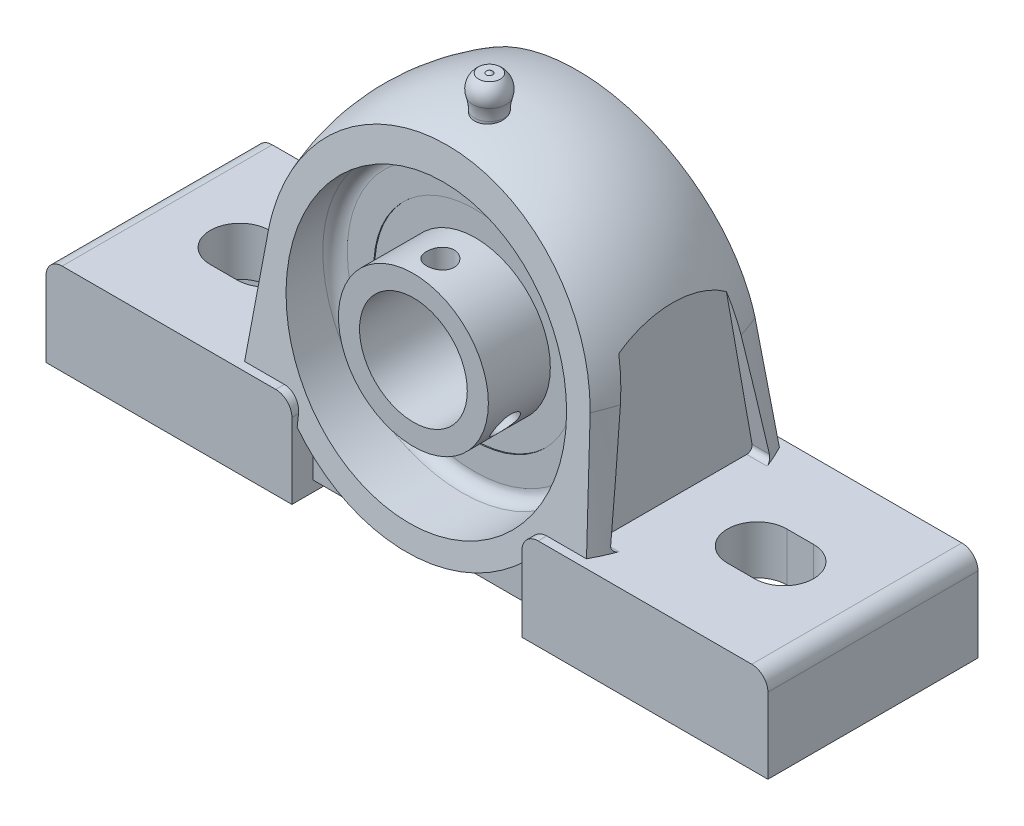
from build123d import *

# Parameters (mm, degrees)
EXTRUDE_984_DEPTH             = 84.85
CUT_EXTRUDE_1_DEPTH           = 55.135249472
CUT_EXTRUDE_1_DEPTH_BACK      = 55.135249472
SKETCH_5_OUTSIDE_W            = 60.452
SKETCH_5_OUTSIDE_H            = 88.062
EXTRUDE_4_REACH               = 60.025
EXTRUDE_4_DIRECTION_2_REACH   = 60.025
EXTRUDE_1_DEPTH               = 19.5
EXTRUDE_1_DEPTH_BACK          = 19.5
CUT_EXTRUDE_3_DEPTH           = 101.761654379
CUT_EXTRUDE_4_DEPTH           = 7.99
CUT_EXTRUDE_4_DRAFT           = -1
CUT_EXTRUDE_4_PROFILE_2_DEPTH = 7.99
CUT_EXTRUDE_4_PROFILE_2_DRAFT = -1
PATTERN_CIRCULAR_1_COUNT      = 12
SKETCH_14_W                   = 31
SKETCH_14_H                   = 3.915
SKETCH_16_W                   = 2.567
SKETCH_16_H                   = 6.115
SKETCH_15_W                   = 0.1
SKETCH_15_H                   = 5.145
PATTERN_CIRCULAR_2_COUNT      = 2
PATTERN_CIRCULAR_2_ANGLE      = 120
CUT_EXTRUDE_START             = 29.81311
CUT_EXTRUDE_5_DEPTH           = 8.58689
CUT_EXTRUDE_START_2           = -38.4
CUT_EXTRUDE_6_DEPTH           = 8.49652


with BuildPart() as part:
    # 草图1 → Extrude 984 (new body)
    with BuildSketch(Plane(origin=(0, -31.3, 0), x_dir=(-1, 0, 0), z_dir=(0, 1, 0))):
        with BuildLine():
            Line((-33.636057661, 18.525), (33.636057661, 18.525))
            ThreePointArc((33.636057661, 18.525), (38.4, 0), (33.636057661, -18.525))
            Line((33.636057661, -18.525), (-33.636057661, -18.525))
            ThreePointArc((-33.636057661, -18.525), (-38.4, 0), (-33.636057661, 18.525))
        make_face()
    extrude(amount=EXTRUDE_984_DEPTH)

    # 切除-扫描1: sweep along a path in 草图3
    with BuildLine(Plane.XY) as sweep_1_path:
        Line((-38.4, -31.3), (-32.994675679, 4.923512654))
        ThreePointArc((-32.994675679, 4.923512654), (0, 33.36), (32.994675679, 4.923512654))
        Line((32.994675679, 4.923512654), (38.4, -31.3))
    # 草图2 → 切除-扫描1 (sweep, cut)
    with BuildSketch(Plane(origin=(0, -31.3, 0), x_dir=(-1, 0, 0), z_dir=(0, 1, 0))):
        with BuildLine():
            Line((-33.636057661, 18.525), (-123.25, 18.525))
            Line((-123.25, 18.525), (-123.25, -18.525))
            Line((-123.25, -18.525), (-33.636057661, -18.525))
            ThreePointArc((-33.636057661, -18.525), (-38.4, 0), (-33.636057661, 18.525))
        make_face()
    sweep(path=sweep_1_path.line, mode=Mode.SUBTRACT)

    # 草图5 outside → 切除-拉伸1 (cut, two sides: drawn at the far end of the back side and taken through both)
    with BuildSketch(Plane(origin=(0, 0, 0), x_dir=(0, 0, -1), z_dir=(1, 0, 0)).offset(-CUT_EXTRUDE_1_DEPTH_BACK)):
        with Locations((0, 1.03)):
            Rectangle(SKETCH_5_OUTSIDE_W, SKETCH_5_OUTSIDE_H)
        Polygon((11.7, 34.36), (18.525, -21.38), (15.6, -21.38), (15.6, -34.3), (-15.6, -34.3), (-15.6, -21.38), (-18.525, -21.38), (-11.7, 34.36), align=None, mode=Mode.SUBTRACT)
    extrude(amount=CUT_EXTRUDE_1_DEPTH + CUT_EXTRUDE_1_DEPTH_BACK, mode=Mode.SUBTRACT)

    # 草图6 → 切除-旋转2 (revolve, cut)
    with BuildSketch(Plane(origin=(0, 0, 0), x_dir=(0, 0, -1), z_dir=(1, 0, 0)), mode=Mode.PRIVATE) as cut_revolve_2_sk:
        with BuildLine():
            Line((-22.565101692, 25.847619048), (-9.277190476, 25.847619048))
            ThreePointArc((-9.277190476, 25.847619048), (-7.666973648, 25.180645399), (-7, 23.570428571))
            Line((-7, 23.570428571), (-7, 22.433234274))
            ThreePointArc((-7, 22.433234274), (-6.069160332, 22.702759587), (-5.128, 22.933678641))
            Line((-5.128, 22.933678641), (-5.128, 25.847619048))
            Line((-5.128, 25.847619048), (-3.256, 25.847619048))
            Line((-3.256, 25.847619048), (-3.256, 23.273342347))
            ThreePointArc((-3.256, 23.273342347), (1.918548773, 23.421553548), (7, 22.433234274))
            Line((7, 22.433234274), (7, 23.570428571))
            ThreePointArc((7, 23.570428571), (7.666973648, 25.180645399), (9.277190476, 25.847619048))
            Line((9.277190476, 25.847619048), (22.565101692, 25.847619048))
            Line((22.565101692, 25.847619048), (25.729974315, 0))
            Line((25.729974315, 0), (-25.729974315, 0))
            Line((-25.729974315, 0), (-22.565101692, 25.847619048))
        make_face()
    revolve(cut_revolve_2_sk.sketch.rotate(Axis((0, 0, 0), (0, 0, -1)), 180), axis=Axis((0, 0, 0), (0, 0, -1)), mode=Mode.SUBTRACT)

    # 草图11 → 凸台-旋转1 (revolve)
    with BuildSketch(Plane.XY.offset(4.192)):
        with BuildLine():
            Line((0, 31.44046273), (0, 39.36))
            ThreePointArc((0, 39.36), (-0.328456711, 39.290107141), (-0.6, 39.092539267))
            Line((-0.6, 39.092539267), (-2, 39.092539267))
            ThreePointArc((-2, 39.092539267), (-3.100653507, 37.504684437), (-3.105555556, 35.572665525))
            ThreePointArc((-3.105555556, 35.572665525), (-2.83938828, 34.406746373), (-2.75, 33.214176785))
            Line((-2.75, 33.214176785), (-2.75, 31.44046273))
            Line((-2.75, 31.44046273), (0, 31.44046273))
        make_face()
    revolve(axis=Axis((0, 0, 4.192), (0, 1, 0)))

    # 凸台-拉伸4: up to this plane
    extrude_4_end = Plane(origin=(-38.4, 34.36, -11.7), z_dir=(0, 0.12153581971911598, -0.9925870463214813))
    # 草图9 → 凸台-拉伸4 (add, up to the surface)
    with BuildSketch(Plane.XY, mode=Mode.PRIVATE) as extrude_4_sk1:
        with BuildLine():
            Line((14.525667297, -21.38), (21.353177431, -21.38))
            ThreePointArc((21.353177431, -21.38), (0, -30.216925496), (-21.353177431, -21.38))
            Line((-21.353177431, -21.38), (-14.525667297, -21.38))
            ThreePointArc((-14.525667297, -21.38), (0, -25.847619048), (14.525667297, -21.38))
        make_face()
    extrude_4_tool1 = split(extrude(extrude_4_sk1.sketch, amount=-EXTRUDE_4_REACH, mode=Mode.PRIVATE), bisect_by=extrude_4_end, keep=Keep.BOTH, mode=Mode.PRIVATE)
    add(extrude_4_tool1.solids().sort_by_distance((0, -25.877182, 0))[0])

    # 凸台-拉伸4 direction 2: up to this plane
    extrude_4_direction_2_end = Plane(origin=(-38.4, 34.36, 11.7), z_dir=(0, 0.12153581971911598, 0.9925870463214813))
    # 草图9 → 凸台-拉伸4 direction 2 (add, up to the surface)
    with BuildSketch(Plane.XY, mode=Mode.PRIVATE) as extrude_4_direction_2_sk1:
        with BuildLine():
            Line((14.525667297, -21.38), (21.353177431, -21.38))
            ThreePointArc((21.353177431, -21.38), (0, -30.216925496), (-21.353177431, -21.38))
            Line((-21.353177431, -21.38), (-14.525667297, -21.38))
            ThreePointArc((-14.525667297, -21.38), (0, -25.847619048), (14.525667297, -21.38))
        make_face()
    extrude_4_direction_2_tool1 = split(extrude(extrude_4_direction_2_sk1.sketch, amount=EXTRUDE_4_DIRECTION_2_REACH, mode=Mode.PRIVATE), bisect_by=extrude_4_direction_2_end, keep=Keep.BOTH, mode=Mode.PRIVATE)
    add(extrude_4_direction_2_tool1.solids().sort_by_distance((0, -25.877182, 0))[0])

    # 草图4 → 凸台-拉伸1 (add, two sides: drawn at the far end of the back side and taken through both)
    with BuildSketch(Plane.XY.offset(-EXTRUDE_1_DEPTH_BACK)):
        with BuildLine():
            Line((24.353177431, -16.3), (64, -16.3))
            ThreePointArc((64, -16.3), (66.121320344, -17.178679656), (67, -19.3))
            Line((67, -19.3), (67, -33.3))
            Line((67, -33.3), (21.353177431, -33.3))
            Line((21.353177431, -33.3), (21.353177431, -19.3))
            ThreePointArc((21.353177431, -19.3), (22.231857088, -17.178679656), (24.353177431, -16.3))
        make_face()
        with BuildLine():
            Line((-64, -16.3), (-24.353177431, -16.3))
            ThreePointArc((-24.353177431, -16.3), (-22.231857088, -17.178679656), (-21.353177431, -19.3))
            Line((-21.353177431, -19.3), (-21.353177431, -33.3))
            Line((-21.353177431, -33.3), (-67, -33.3))
            Line((-67, -33.3), (-67, -19.3))
            ThreePointArc((-67, -19.3), (-66.121320344, -17.178679656), (-64, -16.3))
        make_face()
    extrude(amount=EXTRUDE_1_DEPTH + EXTRUDE_1_DEPTH_BACK)

    # 草图7 → 切除-拉伸3 (cut, through all)
    with BuildSketch(Plane.XZ.offset(33.3)):
        with BuildLine():
            Line((-45.5, 5.5), (-50.5, 5.5))
            ThreePointArc((-50.5, 5.5), (-56, 0), (-50.5, -5.5))
            Line((-50.5, -5.5), (-45.5, -5.5))
            ThreePointArc((-45.5, -5.5), (-40, 0), (-45.5, 5.5))
        make_face()
        with BuildLine():
            Line((45.5, -5.5), (50.5, -5.5))
            ThreePointArc((50.5, -5.5), (56, 0), (50.5, 5.5))
            Line((50.5, 5.5), (45.5, 5.5))
            ThreePointArc((45.5, 5.5), (40, 0), (45.5, -5.5))
        make_face()
    extrude(amount=-CUT_EXTRUDE_3_DEPTH, mode=Mode.SUBTRACT)


with BuildPart() as cut_extrude_4_tool:
    # 草图10 → 切除-拉伸4 (with draft: the straight prism first)
    with BuildSketch(Plane.XZ.offset(33.3)):
        with BuildLine():
            ThreePointArc((50.5, -10.73), (51.015492065, -9.485492065), (52.26, -8.97))
            Line((52.26, -8.97), (59.975, -8.97))
            ThreePointArc((59.975, -8.97), (61.219507935, -8.454507935), (61.735, -7.21))
            Line((61.735, -7.21), (61.735, 7.21))
            ThreePointArc((61.735, 7.21), (61.219507935, 8.454507935), (59.975, 8.97))
            Line((59.975, 8.97), (52.26, 8.97))
            ThreePointArc((52.26, 8.97), (51.015492065, 9.485492065), (50.5, 10.73))
            Line((50.5, 10.73), (50.5, 12.475))
            ThreePointArc((50.5, 12.475), (49.984507935, 13.719507935), (48.74, 14.235))
            Line((48.74, 14.235), (28.378177431, 14.235))
            ThreePointArc((28.378177431, 14.235), (27.133669496, 13.719507935), (26.618177431, 12.475))
            Line((26.618177431, 12.475), (26.618177431, -12.475))
            ThreePointArc((26.618177431, -12.475), (27.133669496, -13.719507935), (28.378177431, -14.235))
            Line((28.378177431, -14.235), (48.74, -14.235))
            ThreePointArc((48.74, -14.235), (49.984507935, -13.719507935), (50.5, -12.475))
            Line((50.5, -12.475), (50.5, -10.73))
        make_face()
    extrude(amount=-CUT_EXTRUDE_4_DEPTH)
    # 切除-拉伸4: the draft: its side faces are tilted about the plane it starts from
    cut_extrude_4_sides = [cut_extrude_4_tool.faces().sort_by_distance(p)[0] for p in [
        (51.015492065, -29.305, -9.485492065),
        (56.1175, -29.305, -8.97),
        (61.219507935, -29.305, -8.454507935),
        (61.735, -29.305, 0),
        (61.219507935, -29.305, 8.454507935),
        (56.1175, -29.305, 8.97),
        (51.015492065, -29.305, 9.485492065),
        (50.5, -29.305, 11.6025),
        (49.984507935, -29.305, 13.719507935),
        (38.559088716, -29.305, 14.235),
        (27.133669496, -29.305, 13.719507935),
        (26.618177431, -29.305, 0),
        (27.133669496, -29.305, -13.719507935),
        (38.559088716, -29.305, -14.235),
        (49.984507935, -29.305, -13.719507935),
        (50.5, -29.305, -11.6025),
    ]]
    draft(cut_extrude_4_sides, Plane.XZ.offset(33.3), CUT_EXTRUDE_4_DRAFT)


with BuildPart() as part_1:
    add(part.part)

    # 切除-拉伸4: cut by cut_extrude_4_tool
    add(cut_extrude_4_tool.part, mode=Mode.SUBTRACT)


with BuildPart() as cut_extrude_4_profile_2_tool:
    # 草图10 → 切除-拉伸4 profile 2 (with draft: the straight prism first)
    with BuildSketch(Plane.XZ.offset(33.3)):
        with BuildLine():
            Line((-59.975, -8.97), (-52.26, -8.97))
            ThreePointArc((-52.26, -8.97), (-51.015492065, -9.485492065), (-50.5, -10.73))
            Line((-50.5, -10.73), (-50.5, -12.475))
            ThreePointArc((-50.5, -12.475), (-49.984507935, -13.719507935), (-48.74, -14.235))
            Line((-48.74, -14.235), (-28.378177431, -14.235))
            ThreePointArc((-28.378177431, -14.235), (-27.133669496, -13.719507935), (-26.618177431, -12.475))
            Line((-26.618177431, -12.475), (-26.618177431, 12.475))
            ThreePointArc((-26.618177431, 12.475), (-27.133669496, 13.719507935), (-28.378177431, 14.235))
            Line((-28.378177431, 14.235), (-48.74, 14.235))
            ThreePointArc((-48.74, 14.235), (-49.984507935, 13.719507935), (-50.5, 12.475))
            Line((-50.5, 12.475), (-50.5, 10.73))
            ThreePointArc((-50.5, 10.73), (-51.015492065, 9.485492065), (-52.26, 8.97))
            Line((-52.26, 8.97), (-59.975, 8.97))
            ThreePointArc((-59.975, 8.97), (-61.219507935, 8.454507935), (-61.735, 7.21))
            Line((-61.735, 7.21), (-61.735, -7.21))
            ThreePointArc((-61.735, -7.21), (-61.219507935, -8.454507935), (-59.975, -8.97))
        make_face()
    extrude(amount=-CUT_EXTRUDE_4_PROFILE_2_DEPTH)
    # 切除-拉伸4 profile 2: the draft: its side faces are tilted about the plane it starts from
    cut_extrude_4_profile_2_sides = [cut_extrude_4_profile_2_tool.faces().sort_by_distance(p)[0] for p in [
        (-56.1175, -29.305, -8.97),
        (-51.015492065, -29.305, -9.485492065),
        (-50.5, -29.305, -11.6025),
        (-49.984507935, -29.305, -13.719507935),
        (-38.559088716, -29.305, -14.235),
        (-27.133669496, -29.305, -13.719507935),
        (-26.618177431, -29.305, 0),
        (-27.133669496, -29.305, 13.719507935),
        (-38.559088716, -29.305, 14.235),
        (-49.984507935, -29.305, 13.719507935),
        (-50.5, -29.305, 11.6025),
        (-51.015492065, -29.305, 9.485492065),
        (-56.1175, -29.305, 8.97),
        (-61.219507935, -29.305, 8.454507935),
        (-61.735, -29.305, 0),
        (-61.219507935, -29.305, -8.454507935),
    ]]
    draft(cut_extrude_4_profile_2_sides, Plane.XZ.offset(33.3), CUT_EXTRUDE_4_PROFILE_2_DRAFT)


with BuildPart() as part_2:
    add(part_1.part)

    # 切除-拉伸4 profile 2: cut by cut_extrude_4_profile_2_tool
    add(cut_extrude_4_profile_2_tool.part, mode=Mode.SUBTRACT)

    # 草图12 → 凸台-旋转3 (revolve)
    with BuildSketch(Plane(origin=(0, 0, 0), x_dir=(0, 0, -1), z_dir=(1, 0, 0)), mode=Mode.PRIVATE) as revolve_3_sk:
        with BuildLine():
            Line((7, 22.453234274), (7, 18.66))
            Line((7, 18.66), (-7, 18.66))
            Line((-7, 18.66), (-7, 22.453234274))
            ThreePointArc((-7, 22.453234274), (0, 23.52), (7, 22.453234274))
        make_face()
    revolve(revolve_3_sk.sketch.rotate(Axis((0, 0, 0), (0, 0, -1)), 180), axis=Axis((0, 0, 0), (0, 0, -1)))

    # 草图13 → 凸台-旋转4 (revolve)
    with BuildSketch(Plane(origin=(0, 0, 0), x_dir=(0, 0, -1), z_dir=(1, 0, 0))):
        with BuildLine():
            Line((0, 20.6175), (0, 12.9225))
            ThreePointArc((0, 12.9225), (3.8475, 16.77), (0, 20.6175))
        make_face()
    revolve_4 = revolve(axis=Axis((0, 0, 0), (0, 1, 0)))

    # 阵列(圆周)1: 凸台-旋转4 ×12 about axis
    pattern_circular_1_axis = Axis((0, 0, 0), (0, 0, 1))
    for i in range(1, PATTERN_CIRCULAR_1_COUNT):
        add(revolve_4.rotate(pattern_circular_1_axis, i * 360 / PATTERN_CIRCULAR_1_COUNT))

    # 草图14 → 凸台-旋转5 (revolve)
    with BuildSketch(Plane(origin=(0, 0, 0), x_dir=(0, 0, -1), z_dir=(1, 0, 0)), mode=Mode.PRIVATE) as revolve_5_sk:
        with Locations((-2.8, 11.9575)):
            Rectangle(SKETCH_14_W, SKETCH_14_H)
    revolve(revolve_5_sk.sketch.rotate(Axis((0, 0, 0), (0, 0, -1)), 90), axis=Axis((0, 0, 0), (0, 0, -1)))

    # 草图16 → 切除-旋转3 (revolve, cut)
    with BuildSketch(Plane(origin=(0, 0, 0), x_dir=(0, 0, -1), z_dir=(1, 0, 0))):
        with Locations((-14.5835, 11.0575)):
            Rectangle(SKETCH_16_W, SKETCH_16_H)
    cut_revolve_3 = revolve(axis=Axis((0, 14.115, 13.3), (0, -1, 0)), mode=Mode.SUBTRACT)

    # 草图15 → 凸台-旋转6 (revolve)
    with BuildSketch(Plane(origin=(0, 0, 0), x_dir=(0, 0, -1), z_dir=(1, 0, 0)), mode=Mode.PRIVATE) as revolve_6_sk:
        with Locations((-6.75, 16.2875)):
            Rectangle(SKETCH_15_W, SKETCH_15_H)
        with Locations((6.75, 16.2875)):
            Rectangle(SKETCH_15_W, SKETCH_15_H)
    revolve(revolve_6_sk.sketch.rotate(Axis((0, 0, 0), (0, 0, -1)), 180), axis=Axis((0, 0, 0), (0, 0, -1)))

    # 阵列(圆周)2: 切除-旋转3 ×2 about axis
    pattern_circular_2_axis = Axis((0, 0, -21.702927371), (0, 0, -1))
    for i in range(1, PATTERN_CIRCULAR_2_COUNT):
        add(cut_revolve_3.rotate(pattern_circular_2_axis, i * PATTERN_CIRCULAR_2_ANGLE / (PATTERN_CIRCULAR_2_COUNT - 1)), mode=Mode.SUBTRACT)

    # 草图17 → 切除-拉伸5 (cut)
    with BuildSketch(Plane(origin=(0, 0, 0), x_dir=(0, 0, -1), z_dir=(1, 0, 0)).offset(CUT_EXTRUDE_START)):
        with BuildLine():
            Line((6.524492273, 31.44046273), (-6.524492273, 31.44046273))
            Line((-6.524492273, 31.44046273), (-14.735478084, -15.126351822))
            ThreePointArc((-14.735478084, -15.126351822), (-14.516714775, -15.94278761), (-13.750670331, -16.3))
            Line((-13.750670331, -16.3), (13.750670331, -16.3))
            ThreePointArc((13.750670331, -16.3), (14.516714775, -15.94278761), (14.735478084, -15.126351822))
            Line((14.735478084, -15.126351822), (6.524492273, 31.44046273))
        make_face()
    extrude(amount=CUT_EXTRUDE_5_DEPTH, mode=Mode.SUBTRACT)

    # 草图17<2> → 切除-拉伸6 (cut)
    with BuildSketch(Plane(origin=(0, 0, 0), x_dir=(0, 0, -1), z_dir=(1, 0, 0)).offset(CUT_EXTRUDE_START_2)):
        with BuildLine():
            Line((6.524492273, 31.44046273), (-6.524492273, 31.44046273))
            Line((-6.524492273, 31.44046273), (-14.735478084, -15.126351822))
            ThreePointArc((-14.735478084, -15.126351822), (-14.516714775, -15.94278761), (-13.750670331, -16.3))
            Line((-13.750670331, -16.3), (13.750670331, -16.3))
            ThreePointArc((13.750670331, -16.3), (14.516714775, -15.94278761), (14.735478084, -15.126351822))
            Line((14.735478084, -15.126351822), (6.524492273, 31.44046273))
        make_face()
    extrude(amount=CUT_EXTRUDE_6_DEPTH, mode=Mode.SUBTRACT)


solid = part_2.part
